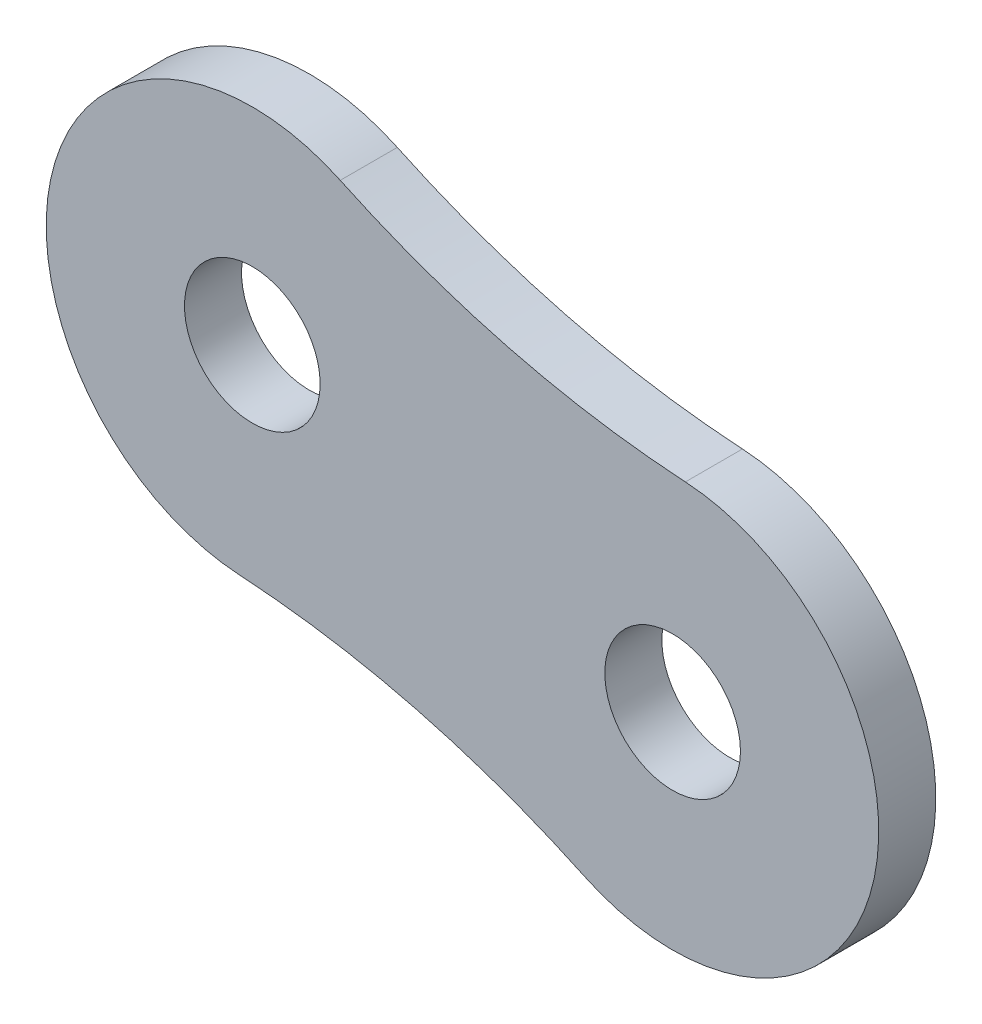
from build123d import *

# Parameters (mm, degrees)
SKETCH_2_R        = 7.94
EXTRUDE_1_DEPTH   = 7.875
EXTRUDE_1_2_DEPTH = 7.875
EXTRUDE_2_DEPTH   = 3.43
SKETCH_6_R        = 3.97
EXTRUDE_4_DEPTH   = 3.34
SCALE_1_SCALE     = 0.65


with BuildPart() as part:
    # 草图2 → 拉伸1 (new, symmetric)
    with BuildSketch(Plane.XY):
        with Locations((12.7, 0)):
            Circle(SKETCH_2_R)
    extrude(amount=EXTRUDE_1_DEPTH, both=True)



with BuildPart() as body_2:
    # 草图2 → Extrude 1 2 (new, symmetric)
    with BuildSketch(Plane.XY):
        with Locations((-12.7, 0)):
            Circle(SKETCH_2_R)
    extrude(amount=EXTRUDE_1_2_DEPTH, both=True)


with BuildPart() as part_1:
    add(part.part)

    add(body_2.part)  # 拉伸2 merges body 2
    # 草图3 → 拉伸2 (add)
    with BuildSketch(Plane.XY.offset(7.875)):
        with BuildLine():
            ThreePointArc((-10.428153415, 11.849174574), (-24.765, 0), (-10.428153415, -11.849174574))
            ThreePointArc((-10.428153415, -11.849174574), (0, -10.8585), (10.428153415, -11.849174574))
            ThreePointArc((10.428153415, -11.849174574), (24.765, 0), (10.428153415, 11.849174574))
            ThreePointArc((10.428153415, 11.849174574), (0, 10.8585), (-10.428153415, 11.849174574))
        make_face()
    extrude(amount=EXTRUDE_2_DEPTH)


with BuildPart() as body_2_2:
    # 草图6 → 拉伸4 (new body)
    with BuildSketch(Plane.XY.offset(11.305)):
        with BuildLine():
            ThreePointArc((32.154770058, -17.228648829), (48.987968132, -9.317166623), (38.048309834, 5.725173103))
            ThreePointArc((38.048309834, 5.725173103), (27.701405286, 7.358998688), (17.847242234, 10.911925695))
            ThreePointArc((17.847242234, 10.911925695), (1.014044161, 3.000443489), (11.953702459, -12.041896237))
            ThreePointArc((11.953702459, -12.041896237), (22.300607007, -13.675721822), (32.154770058, -17.228648829))
        make_face()
        with Locations((12.7, 0)):
            Circle(SKETCH_6_R, mode=Mode.SUBTRACT)
        with Locations((37.302012293, -6.316723134)):
            Circle(SKETCH_6_R, mode=Mode.SUBTRACT)
    extrude(amount=EXTRUDE_4_DEPTH)


with BuildPart() as body_2_2_1:
    # 缩放比例1: scaled about (0, 0, 0)
    add(body_2_2.part.scale(SCALE_1_SCALE))


solid = body_2_2_1.part
